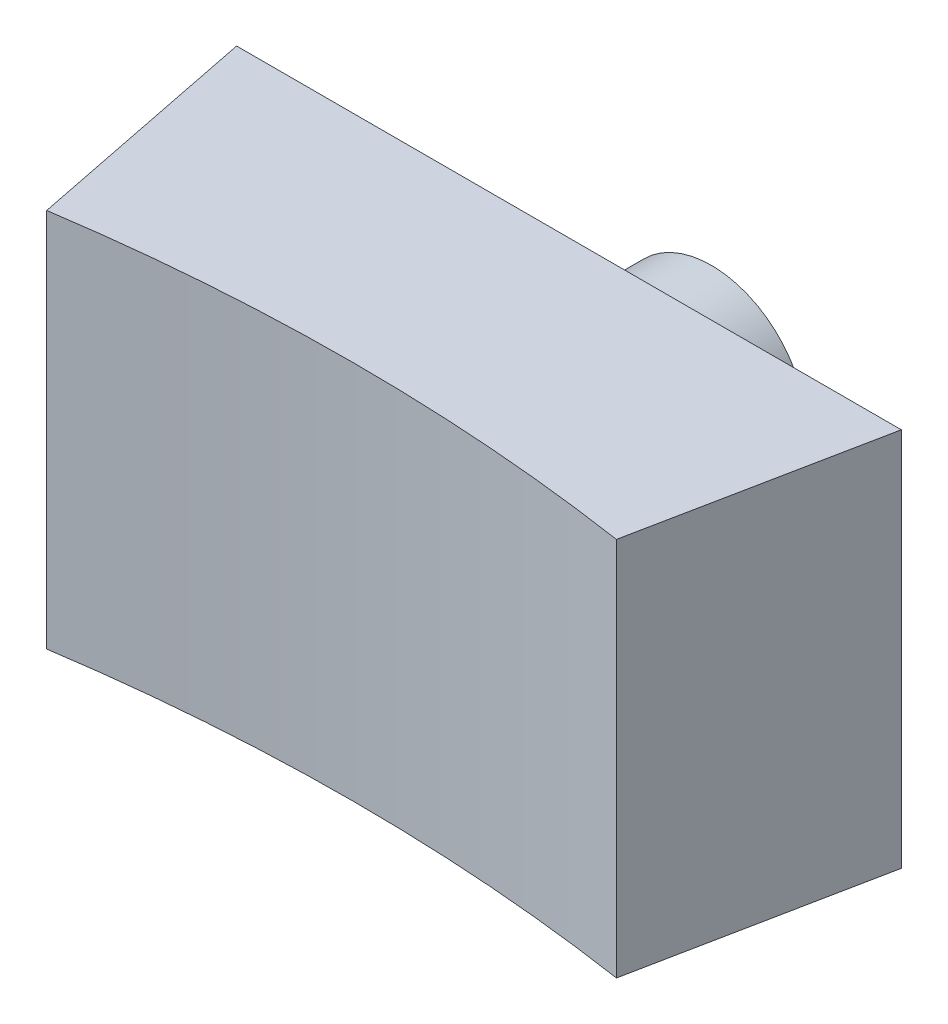
SolidWorks part; units mm, degrees
ref_plane "Front Plane" through (0, 0, 0) normal (0, 0, 1) x (1, 0, 0)
ref_plane "Top Plane" through (0, 0, 0) normal (0, 1, 0) x (1, 0, 0)
ref_plane "Right Plane" through (0, 0, 0) normal (1, 0, 0) x (0, 0, -1)
sketch "Sketch1" plane through (0, 0, 0) normal (0, 1, 0) x (1, 0, 0)
  line L0 (7, 0) -> (-7, 0)
  line L1 (-7, 0) -> (-6, -5)
  line L2 (0, 36.6957) -> (0, -57.2174) construction
  line L3 (7, 0) -> (6, -5)
  arc A0 (-6, -5) -> (6, -5) centre (0, -44.5474) cw
  dimension "D4" = 40
  dimension "D1" = 5
  dimension "D2" = 14
  dimension "D3" = 12
extrude "Boss-Extrude1" add sketch "Sketch1" along normal mid plane 8
sketch "Sketch2" plane through (0, 0, 0) normal (0, 0, 1) x (1, 0, 0)
  circle A0 centre (0, 0) radius 1.5
  circle A1 centre (0, 0) radius 2
  dimension "D1" = 3
  dimension "D2" = 4
extrude "Boss-Extrude2" add sketch "Sketch2" against normal blind 3
